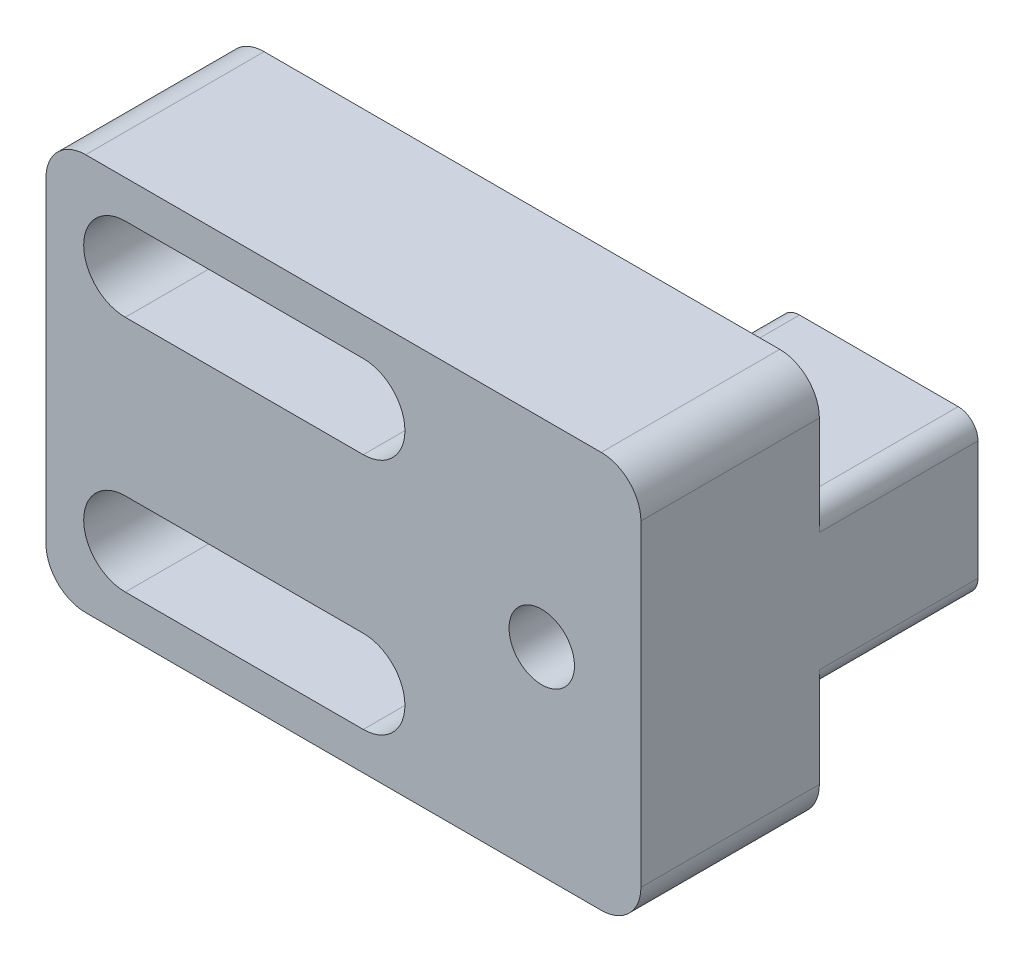
from build123d import *

# Parameters (mm, degrees)
SKETCH_1_W          = 10
SKETCH_1_H          = 8
EXTRUDE_1_DEPTH     = 8
SKETCH_2_W          = 10
SKETCH_2_H          = 20
EXTRUDE_2_DEPTH     = 9
SKETCH_4_R          = 1.65
CUT_EXTRUDE_2_DEPTH = 6
SKETCH_7_W          = 9
SKETCH_7_H          = 20
EXTRUDE_3_DEPTH     = 20
CUT_EXTRUDE_5_DEPTH = 20
FILLET_2_R          = 2
FILLET_3_R          = 1


with BuildPart() as part:
    # 草图1 → 凸台-拉伸1 (new body)
    with BuildSketch(Plane.XY):
        Rectangle(SKETCH_1_W, SKETCH_1_H)
    extrude(amount=EXTRUDE_1_DEPTH)

    # 草图2 → 凸台-拉伸2 (add)
    with BuildSketch(Plane.XY.offset(8)):
        Rectangle(SKETCH_2_W, SKETCH_2_H)
    extrude(amount=EXTRUDE_2_DEPTH)

    # 草图4 → 切除-拉伸2 (cut)
    with BuildSketch(Plane.XY.offset(17)):
        Circle(SKETCH_4_R)
    extrude(amount=-CUT_EXTRUDE_2_DEPTH, mode=Mode.SUBTRACT)

    # 草图7 → 凸台-拉伸3 (add)
    with BuildSketch(Plane.ZY.offset(5)):
        with Locations((12.5, 0)):
            Rectangle(SKETCH_7_W, SKETCH_7_H)
    extrude(amount=EXTRUDE_3_DEPTH)

    # 草图8 → 切除-拉伸5 (cut)
    with BuildSketch(Plane.XY.offset(17)):
        with BuildLine():
            Line((-21, 8.1), (-9, 8.1))
            ThreePointArc((-9, 8.1), (-6.9, 6), (-9, 3.9))
            Line((-9, 3.9), (-21, 3.9))
            ThreePointArc((-21, 3.9), (-23.1, 6), (-21, 8.1))
        make_face()
        with BuildLine():
            Line((-21, -8.1), (-9, -8.1))
            ThreePointArc((-9, -8.1), (-6.9, -6), (-9, -3.9))
            Line((-9, -3.9), (-21, -3.9))
            ThreePointArc((-21, -3.9), (-23.1, -6), (-21, -8.1))
        make_face()
    extrude(amount=-CUT_EXTRUDE_5_DEPTH, mode=Mode.SUBTRACT)

    # 圆角2
    fillet_2_edges = [part.edges().sort_by_distance(p)[0] for p in [
        (5, -10, 12.5),
        (5, 10, 12.5),
        (-25, -10, 12.5),
        (-25, 10, 12.5),
    ]]
    fillet(fillet_2_edges, radius=FILLET_2_R)

    # 圆角3
    fillet_3_edges = [part.edges().sort_by_distance(p)[0] for p in [
        (5, -4, 4),
        (-5, -4, 4),
        (-5, 4, 4),
        (5, 4, 4),
    ]]
    fillet(fillet_3_edges, radius=FILLET_3_R)


solid = part.part
